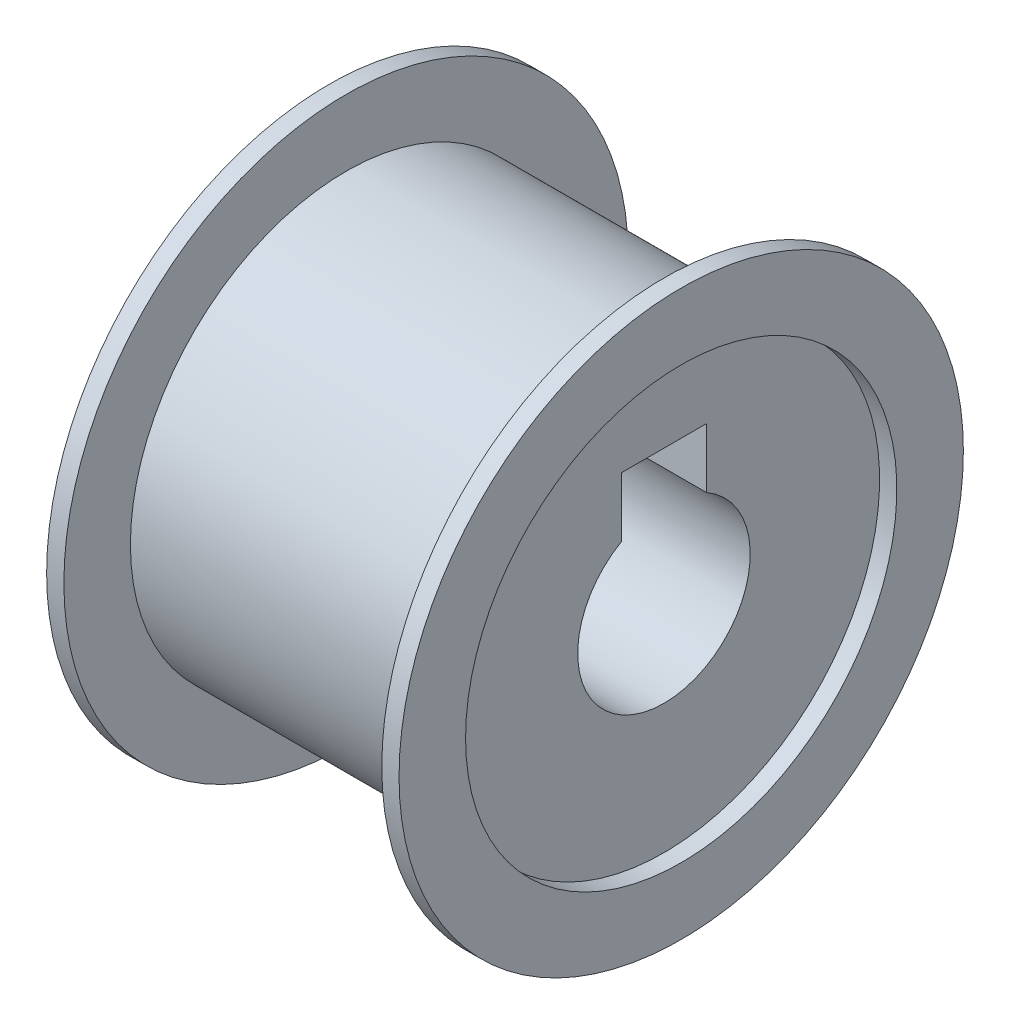
from build123d import *

# Parameters (mm, degrees)
SKETCH1_W          = 3.685714286
SKETCH1_H          = 1.5
SKETCH1_W_2        = 0.2
SKETCH1_H_2        = 0.771428571
CUT_EXTRUDE1_START = -10
CUT_EXTRUDE1_DEPTH = 10


with BuildPart() as part:
    # Sketch1 → Revolve1 (revolve)
    with BuildSketch(Plane(origin=(0, 0, 0), x_dir=(1, 0, 0), z_dir=(0, 1, 0)), mode=Mode.PRIVATE) as revolve1_sk:
        with Locations((0, 1.75)):
            Rectangle(SKETCH1_W, SKETCH1_H)
        with Locations((1.942857143, 2.885714286)):
            Rectangle(SKETCH1_W_2, SKETCH1_H_2)
        with Locations((-1.942857143, 2.885714286)):
            Rectangle(SKETCH1_W_2, SKETCH1_H_2)
    revolve(revolve1_sk.sketch.rotate(Axis((0, 0, 0), (1, 0, 0)), 180), axis=Axis((0, 0, 0), (1, 0, 0)))

    # Sketch2 → Cut-Extrude1 (cut)
    with BuildSketch(Plane.ZY.offset(1.842857143).offset(CUT_EXTRUDE1_START)):
        with BuildLine():
            ThreePointArc((-0.494712466, 0.869056716), (0, 1), (0.494712466, 0.869056716))
            Line((0.494712466, 0.869056716), (0.494712466, 1.562249891))
            Line((0.494712466, 1.562249891), (-0.494712466, 1.562249891))
            Line((-0.494712466, 1.562249891), (-0.494712466, 0.869056716))
        make_face()
    extrude(amount=CUT_EXTRUDE1_DEPTH, mode=Mode.SUBTRACT)


solid = part.part
